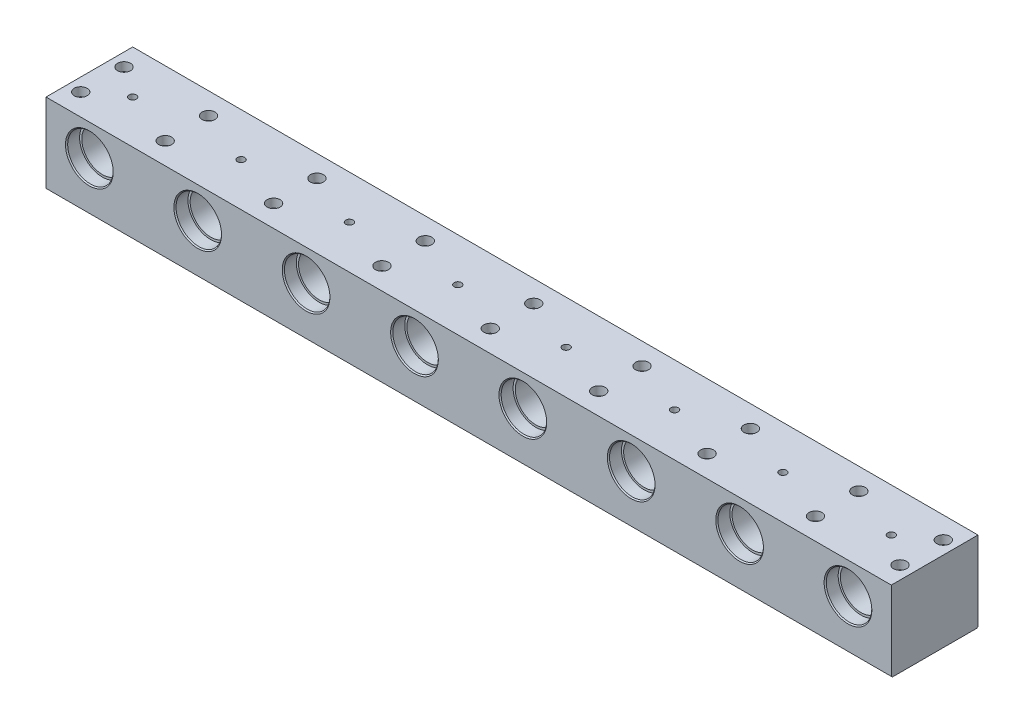
from build123d import *

# Parameters (mm, degrees)
SKETCH2_W                    = 80
SKETCH2_H                    = 74
BOSS_EXTRUDE1_DEPTH          = 390
SKETCH3_R                    = 21
CUT_EXTRUDE1_DEPTH           = 12
SKETCH4_R                    = 19
CUT_EXTRUDE2_DEPTH           = 398.609104524
CHAMFER1_SIZE                = 1
LPATTERN1_COUNT              = 8
LPATTERN1_PITCH              = 100
LPATTERN1_COPY_1_SKETCH_R    = 21
LPATTERN1_COPY_1_DEPTH       = 12
LPATTERN1_COPY_2_SKETCH_R    = 21
LPATTERN1_COPY_2_DEPTH       = 12
LPATTERN1_COPY_3_SKETCH_R    = 21
LPATTERN1_COPY_3_DEPTH       = 12
LPATTERN1_COPY_4_SKETCH_R    = 21
LPATTERN1_COPY_4_DEPTH       = 12
LPATTERN1_COPY_5_SKETCH_R    = 21
LPATTERN1_COPY_5_DEPTH       = 12
LPATTERN1_COPY_6_SKETCH_R    = 21
LPATTERN1_COPY_6_DEPTH       = 12
LPATTERN1_COPY_7_SKETCH_R    = 21
LPATTERN1_COPY_7_DEPTH       = 12
CHAMFER1_OF_LPATTERN1_SIZE   = 1
HOLE1_D                      = 8
HOLE1_CBORE_D                = 12
HOLE1_CBORE_DEPTH            = 8
LPATTERN2_COUNT              = 7
LPATTERN2_PITCH              = 100
LPATTERN2_COPY_1_D           = 8
LPATTERN2_COPY_1_CBORE_D     = 12
LPATTERN2_COPY_1_CBORE_DEPTH = 8
LPATTERN2_COPY_2_D           = 8
LPATTERN2_COPY_2_CBORE_D     = 12
LPATTERN2_COPY_2_CBORE_DEPTH = 8
LPATTERN2_COPY_3_D           = 8
LPATTERN2_COPY_3_CBORE_D     = 12
LPATTERN2_COPY_3_CBORE_DEPTH = 8
LPATTERN2_COPY_4_D           = 8
LPATTERN2_COPY_4_CBORE_D     = 12
LPATTERN2_COPY_4_CBORE_DEPTH = 8
LPATTERN2_COPY_5_D           = 8
LPATTERN2_COPY_5_CBORE_D     = 12
LPATTERN2_COPY_5_CBORE_DEPTH = 8
LPATTERN2_COPY_6_D           = 8
LPATTERN2_COPY_6_CBORE_D     = 12
LPATTERN2_COPY_6_CBORE_DEPTH = 8
LPATTERN3_COUNT              = 8
LPATTERN3_PITCH              = 100
CHAMFER2_SIZE                = 1
HOLE2_D                      = 8
HOLE2_CBORE_D                = 12
HOLE2_CBORE_DEPTH            = 8
MIRROR6_COPY_1_D             = 8
MIRROR6_COPY_1_CBORE_D       = 12
MIRROR6_COPY_1_CBORE_DEPTH   = 8


with BuildPart() as part:
    # Sketch2 → Boss-Extrude1 (new, symmetric)
    with BuildSketch(Plane(origin=(0, 0, 0), x_dir=(0, 0, -1), z_dir=(1, 0, 0))):
        Rectangle(SKETCH2_W, SKETCH2_H)
    extrude(amount=BOSS_EXTRUDE1_DEPTH, both=True)

    # Sketch3 → Cut-Extrude1 (cut)
    with BuildSketch(Plane.XY.offset(40)):
        with Locations((-350, 8)):
            Circle(SKETCH3_R)
    cut_extrude1 = extrude(amount=-CUT_EXTRUDE1_DEPTH, mode=Mode.SUBTRACT)

    # Mirror1: Cut-Extrude1 across plane
    add(cut_extrude1.mirror(Plane.XY), mode=Mode.SUBTRACT)

    # Sketch4 → Cut-Extrude2 (cut, through all)
    with BuildSketch(Plane.XY.offset(28)):
        with Locations((-350, 8)):
            Circle(SKETCH4_R)
    cut_extrude2 = extrude(amount=-CUT_EXTRUDE2_DEPTH, mode=Mode.SUBTRACT)

    # Chamfer1
    chamfer1_edges = [part.edges().sort_by_distance(p)[0] for p in [
        (-371, 8, 40),
        (-371, 8, -40),
    ]]
    chamfer(chamfer1_edges, length=CHAMFER1_SIZE)

    # LPattern1: Cut-Extrude1, Cut-Extrude2 ×8
    with Locations(*[(i * LPATTERN1_PITCH, 0, 0) for i in range(1, LPATTERN1_COUNT)]):
        add(cut_extrude1, mode=Mode.SUBTRACT)
        add(cut_extrude2, mode=Mode.SUBTRACT)

    # LPattern1 copy 1 sketch → LPattern1 copy 1 (cut)
    with BuildSketch(Plane(origin=(100, 0, -40), x_dir=(1, 0, 0), z_dir=(0, 0, -1))):
        with Locations((-350, -8)):
            Circle(LPATTERN1_COPY_1_SKETCH_R)
    extrude(amount=-LPATTERN1_COPY_1_DEPTH, mode=Mode.SUBTRACT)

    # LPattern1 copy 2 sketch → LPattern1 copy 2 (cut)
    with BuildSketch(Plane(origin=(200, 0, -40), x_dir=(1, 0, 0), z_dir=(0, 0, -1))):
        with Locations((-350, -8)):
            Circle(LPATTERN1_COPY_2_SKETCH_R)
    extrude(amount=-LPATTERN1_COPY_2_DEPTH, mode=Mode.SUBTRACT)

    # LPattern1 copy 3 sketch → LPattern1 copy 3 (cut)
    with BuildSketch(Plane(origin=(300, 0, -40), x_dir=(1, 0, 0), z_dir=(0, 0, -1))):
        with Locations((-350, -8)):
            Circle(LPATTERN1_COPY_3_SKETCH_R)
    extrude(amount=-LPATTERN1_COPY_3_DEPTH, mode=Mode.SUBTRACT)

    # LPattern1 copy 4 sketch → LPattern1 copy 4 (cut)
    with BuildSketch(Plane(origin=(400, 0, -40), x_dir=(1, 0, 0), z_dir=(0, 0, -1))):
        with Locations((-350, -8)):
            Circle(LPATTERN1_COPY_4_SKETCH_R)
    extrude(amount=-LPATTERN1_COPY_4_DEPTH, mode=Mode.SUBTRACT)

    # LPattern1 copy 5 sketch → LPattern1 copy 5 (cut)
    with BuildSketch(Plane(origin=(500, 0, -40), x_dir=(1, 0, 0), z_dir=(0, 0, -1))):
        with Locations((-350, -8)):
            Circle(LPATTERN1_COPY_5_SKETCH_R)
    extrude(amount=-LPATTERN1_COPY_5_DEPTH, mode=Mode.SUBTRACT)

    # LPattern1 copy 6 sketch → LPattern1 copy 6 (cut)
    with BuildSketch(Plane(origin=(600, 0, -40), x_dir=(1, 0, 0), z_dir=(0, 0, -1))):
        with Locations((-350, -8)):
            Circle(LPATTERN1_COPY_6_SKETCH_R)
    extrude(amount=-LPATTERN1_COPY_6_DEPTH, mode=Mode.SUBTRACT)

    # LPattern1 copy 7 sketch → LPattern1 copy 7 (cut)
    with BuildSketch(Plane(origin=(700, 0, -40), x_dir=(1, 0, 0), z_dir=(0, 0, -1))):
        with Locations((-350, -8)):
            Circle(LPATTERN1_COPY_7_SKETCH_R)
    extrude(amount=-LPATTERN1_COPY_7_DEPTH, mode=Mode.SUBTRACT)

    # Chamfer1 of LPattern1
    chamfer1_of_lpattern1_edges = [part.edges().sort_by_distance(p)[0] for p in [
        (-271, 8, 40),
        (-271, 8, -40),
        (-171, 8, 40),
        (-171, 8, -40),
        (-71, 8, 40),
        (-71, 8, -40),
        (29, 8, 40),
        (29, 8, -40),
        (129, 8, 40),
        (129, 8, -40),
        (229, 8, 40),
        (229, 8, -40),
        (329, 8, 40),
        (329, 8, -40),
    ]]
    chamfer(chamfer1_of_lpattern1_edges, length=CHAMFER1_OF_LPATTERN1_SIZE)

    # Hole1 (through all)
    with Locations(Plane(origin=(0, 37, 0), x_dir=(1, 0, 0), z_dir=(0, 1, 0))):
        with Locations((-300, 20)):
            hole1 = CounterBoreHole(HOLE1_D / 2, HOLE1_CBORE_D / 2, HOLE1_CBORE_DEPTH)

    # Mirror4: Hole1 across plane
    add(hole1.mirror(Plane.XY), mode=Mode.SUBTRACT)

    # LPattern2: Hole1 ×7
    with Locations(*[(i * LPATTERN2_PITCH, 0, 0) for i in range(1, LPATTERN2_COUNT)]):
        add(hole1, mode=Mode.SUBTRACT)

    # LPattern2 copy 1 (through all)
    with Locations(Plane(origin=(100, 37, 0), x_dir=(1, 0, 0), z_dir=(0, 1, 0))):
        with Locations((-300, -20)):
            CounterBoreHole(LPATTERN2_COPY_1_D / 2, LPATTERN2_COPY_1_CBORE_D / 2, LPATTERN2_COPY_1_CBORE_DEPTH)

    # LPattern2 copy 2 (through all)
    with Locations(Plane(origin=(200, 37, 0), x_dir=(1, 0, 0), z_dir=(0, 1, 0))):
        with Locations((-300, -20)):
            CounterBoreHole(LPATTERN2_COPY_2_D / 2, LPATTERN2_COPY_2_CBORE_D / 2, LPATTERN2_COPY_2_CBORE_DEPTH)

    # LPattern2 copy 3 (through all)
    with Locations(Plane(origin=(300, 37, 0), x_dir=(1, 0, 0), z_dir=(0, 1, 0))):
        with Locations((-300, -20)):
            CounterBoreHole(LPATTERN2_COPY_3_D / 2, LPATTERN2_COPY_3_CBORE_D / 2, LPATTERN2_COPY_3_CBORE_DEPTH)

    # LPattern2 copy 4 (through all)
    with Locations(Plane(origin=(400, 37, 0), x_dir=(1, 0, 0), z_dir=(0, 1, 0))):
        with Locations((-300, -20)):
            CounterBoreHole(LPATTERN2_COPY_4_D / 2, LPATTERN2_COPY_4_CBORE_D / 2, LPATTERN2_COPY_4_CBORE_DEPTH)

    # LPattern2 copy 5 (through all)
    with Locations(Plane(origin=(500, 37, 0), x_dir=(1, 0, 0), z_dir=(0, 1, 0))):
        with Locations((-300, -20)):
            CounterBoreHole(LPATTERN2_COPY_5_D / 2, LPATTERN2_COPY_5_CBORE_D / 2, LPATTERN2_COPY_5_CBORE_DEPTH)

    # LPattern2 copy 6 (through all)
    with Locations(Plane(origin=(600, 37, 0), x_dir=(1, 0, 0), z_dir=(0, 1, 0))):
        with Locations((-300, -20)):
            CounterBoreHole(LPATTERN2_COPY_6_D / 2, LPATTERN2_COPY_6_CBORE_D / 2, LPATTERN2_COPY_6_CBORE_DEPTH)

    # Sketch12 → M8 Tapped Hole1 (revolve, cut)
    with BuildSketch(Plane(origin=(-350, 37, 0), x_dir=(0, 0, 1), z_dir=(1, 0, 0))):
        Polygon((0, 0), (0, 21.792926105), (3.4, 19.75), (3.4, 0), align=None)
    m8_tapped_hole1 = revolve(axis=Axis((-350, 43.35, 0), (0, -1, 0)), mode=Mode.SUBTRACT)

    # LPattern3: M8 Tapped Hole1 ×8
    with Locations(*[(i * LPATTERN3_PITCH, 0, 0) for i in range(1, LPATTERN3_COUNT)]):
        add(m8_tapped_hole1, mode=Mode.SUBTRACT)

    # Chamfer2
    chamfer2_edges = [part.edges().sort_by_distance(p)[0] for p in [
        (0, -37, -40),
        (0, -37, 40),
    ]]
    chamfer(chamfer2_edges, length=CHAMFER2_SIZE)

    # Hole2 (through all)
    with Locations(Plane(origin=(0, 37, 0), x_dir=(1, 0, 0), z_dir=(0, 1, 0))):
        with Locations((-378, 20)):
            hole2 = CounterBoreHole(HOLE2_D / 2, HOLE2_CBORE_D / 2, HOLE2_CBORE_DEPTH)

    # Mirror5: Hole2 across plane
    add(hole2.mirror(Plane.XY), mode=Mode.SUBTRACT)

    # Mirror6: Hole2 across plane
    add(hole2.mirror(Plane(origin=(0, 0, 0), x_dir=(0, 0, 1), z_dir=(1, 0, 0))), mode=Mode.SUBTRACT)

    # Mirror6 copy 1 (through all)
    with Locations(Plane(origin=(0, 37, 0), x_dir=(-1, 0, 0), z_dir=(0, 1, 0))):
        with Locations((-378, 20)):
            CounterBoreHole(MIRROR6_COPY_1_D / 2, MIRROR6_COPY_1_CBORE_D / 2, MIRROR6_COPY_1_CBORE_DEPTH)


solid = part.part
